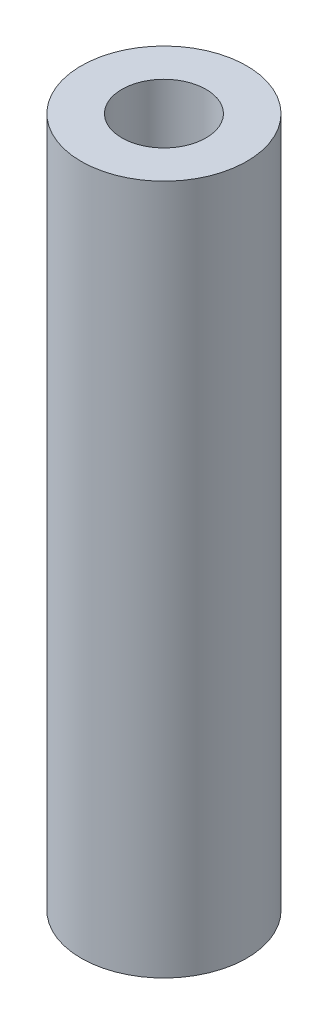
from build123d import *

# Parameters (mm, degrees)
SKETCH1_R           = 6
SKETCH1_R_2         = 3.05
BOSS_EXTRUDE1_DEPTH = 50


with BuildPart() as part:
    # Sketch1 → Boss-Extrude1 (new body)
    with BuildSketch(Plane(origin=(0, 0, 0), x_dir=(1, 0, 0), z_dir=(0, 1, 0))):
        with Locations(Location((0, 0, 0), (0, 0, 270))):
            Circle(SKETCH1_R)
        with Locations(Location((0, 0, 0), (0, 0, 270))):
            Circle(SKETCH1_R_2, mode=Mode.SUBTRACT)
    extrude(amount=BOSS_EXTRUDE1_DEPTH)


solid = part.part
